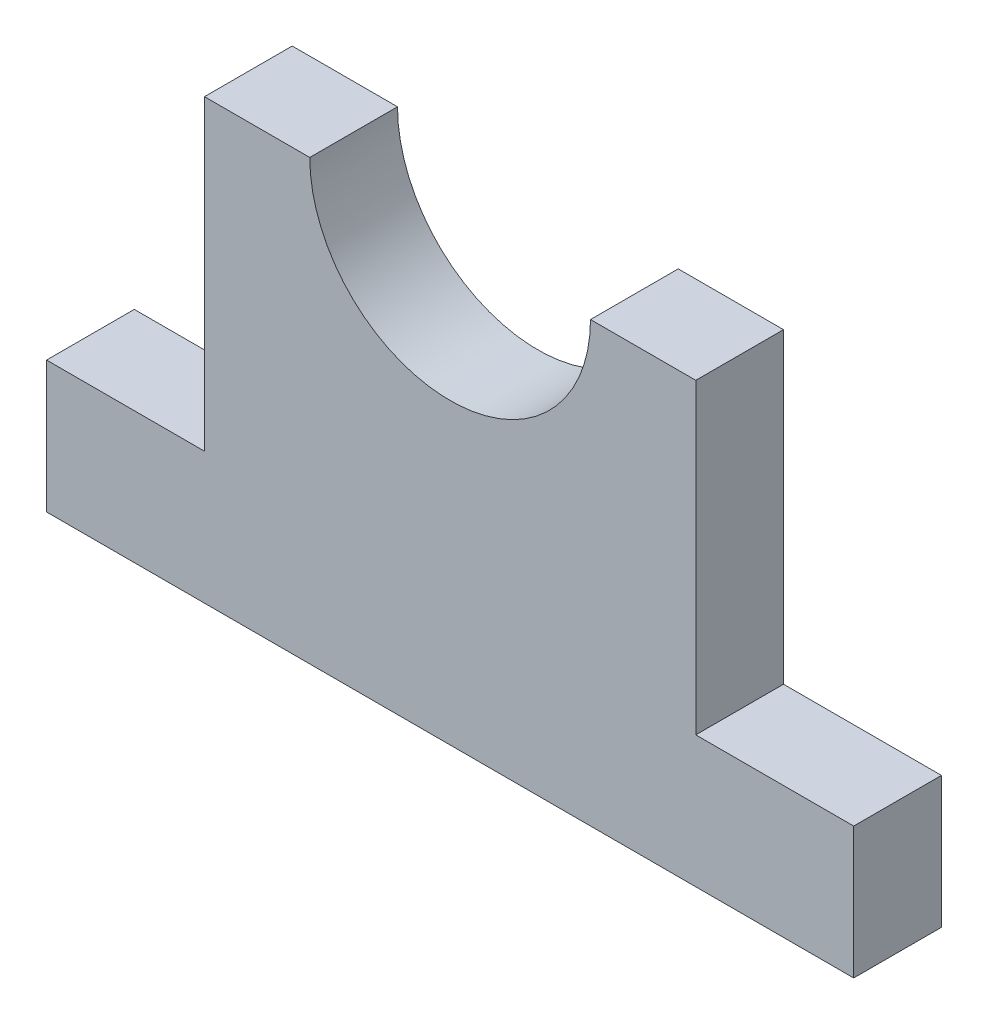
SolidWorks part; units mm, degrees
ref_plane "Front Plane" through (0, 0, 0) normal (0, 0, 1) x (1, 0, 0)
ref_plane "Top Plane" through (0, 0, 0) normal (0, 1, 0) x (1, 0, 0)
ref_plane "Right Plane" through (0, 0, 0) normal (1, 0, 0) x (0, 0, -1)
other "Configuration Table"
sketch "Sketch1" plane through (0, 0, 0) normal (0, 0, 1) x (1, 0, 0)
  line L0 (-16, 50) -> (-28, 50)
  line L1 (-28, 50) -> (-28, 15)
  line L2 (-28, 15) -> (-46, 15)
  line L3 (-46, 15) -> (-46, 0)
  line L4 (-46, 0) -> (46, 0)
  line L5 (0, 0) -> (0, 34) construction
  line L6 (46, 15) -> (46, 0)
  line L7 (28, 15) -> (46, 15)
  line L8 (28, 50) -> (28, 15)
  line L9 (16, 50) -> (28, 50)
  arc A0 (-16, 50) -> (16, 50) centre (0, 50) ccw
  dimension "D1" = 32
  dimension "D2" = 50
  dimension "D3" = 15
  dimension "D4" = 12
  dimension "D5" = 18
extrude "Boss-Extrude1" add sketch "Sketch1" along normal blind 10
